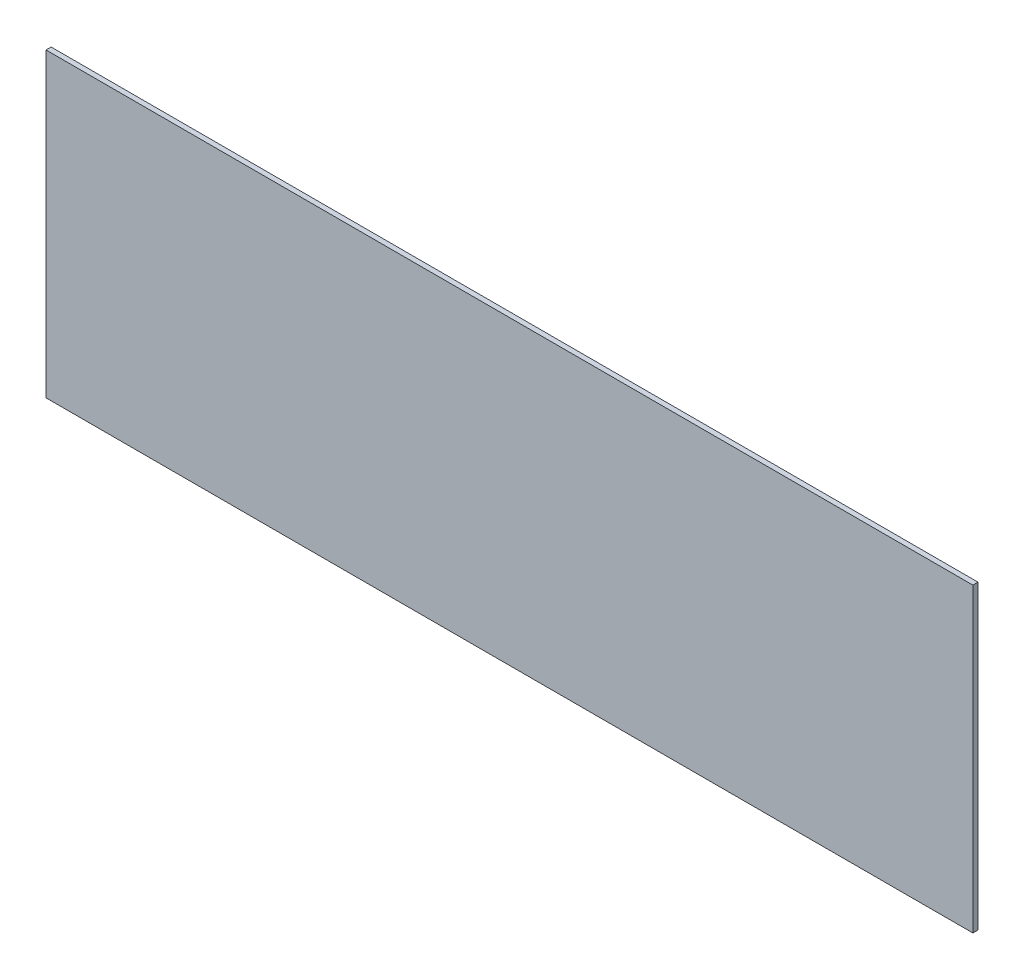
SolidWorks part; units mm, degrees
material "有机玻璃 (PMMA)"
ref_plane "前视" through (0, 0, 0) normal (0, 0, 1) x (1, 0, 0)
ref_plane "上视" through (0, 0, 0) normal (0, 1, 0) x (1, 0, 0)
ref_plane "右视" through (0, 0, 0) normal (1, 0, 0) x (0, 0, -1)
sketch "草图1" plane through (0, 0, 0) normal (0, 0, 1) x (1, 0, 0)
  line L1 (-363, 118) -> (363, 118)
  line L2 (-363, 118) -> (-363, -118)
  line L3 (-363, -118) -> (363, -118)
  line L4 (363, 118) -> (363, -118)
  line L5 (-363, 118) -> (363, -118) construction
  line L6 (-363, -118) -> (363, 118) construction
  point P0 (0, 0)
  dimension "D1" = 726
  dimension "D2" = 236
extrude "凸台-拉伸1" add sketch "草图1" along normal blind 4
